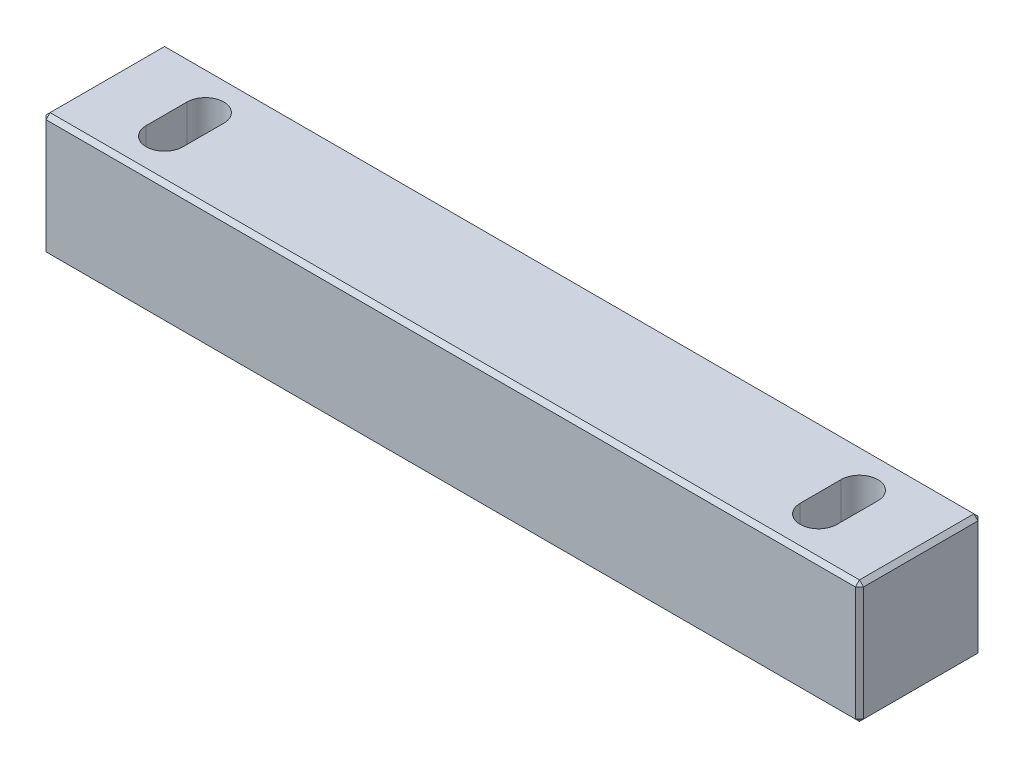
SolidWorks part; units mm, degrees
material "45#"
ref_plane "Front Plane" through (0, 0, 0) normal (0, 0, 1) x (1, 0, 0)
ref_plane "Top Plane" through (0, 0, 0) normal (0, 1, 0) x (1, 0, 0)
ref_plane "Right Plane" through (0, 0, 0) normal (1, 0, 0) x (0, 0, -1)
sketch "Sketch1" plane through (0, 0, 0) normal (0, 1, 0) x (1, 0, 0)
  line L0 (-50, 7.5) -> (50, -7.5) construction
  line L1 (-50, 7.5) -> (50, 7.5)
  line L2 (-50, 7.5) -> (-50, -7.5)
  line L3 (-50, -7.5) -> (50, -7.5)
  line L4 (50, 7.5) -> (50, -7.5)
  dimension "D1" = 100
  dimension "D2" = 15
extrude "Extrude1" add sketch "Sketch1" along normal blind 15
sketch "Sketch4" plane through (0, 15, 0) normal (0, 1, 0) x (1, 0, 0)
  line L0 (0, 7.5) -> (0, -7.5) construction
  line L1 (50, 7.5) -> (-50, 7.5) construction
  line L2 (-42.25, 2.5) -> (-42.25, -2.5)
  line L3 (-50, -7.5) -> (50, -7.5) construction
  line L4 (-37.75, 2.5) -> (-37.75, -2.5)
  line L5 (37.75, 2.5) -> (37.75, -2.5)
  line L6 (-37.75, 0) -> (0, 0) construction
  line L7 (42.25, 2.5) -> (42.25, -2.5)
  arc A0 (-42.25, 2.5) -> (-37.75, 2.5) centre (-40, 2.5) cw
  arc A1 (-37.75, -2.5) -> (-42.25, -2.5) centre (-40, -2.5) cw
  arc A2 (37.75, -2.5) -> (42.25, -2.5) centre (40, -2.5) ccw
  arc A3 (42.25, 2.5) -> (37.75, 2.5) centre (40, 2.5) ccw
  dimension "D3" = 80
  dimension "D1" = 4.5
  dimension "D2" = 5
extrude "Cut-Extrude1" cut sketch "Sketch4" against normal through all
chamfer "Chamfer1" distance 0.5 angle 45 12 edges at (-50, 0, 0) (-50, 7.5, -7.5) (0, 0, -7.5) (50, 7.5, -7.5) (50, 0, 0) (-50, 7.5, 7.5) (0, 0, 7.5) (50, 7.5, 7.5) (0, 15, -7.5) (50, 15, 0) (0, 15, 7.5) (-50, 15, 0)
